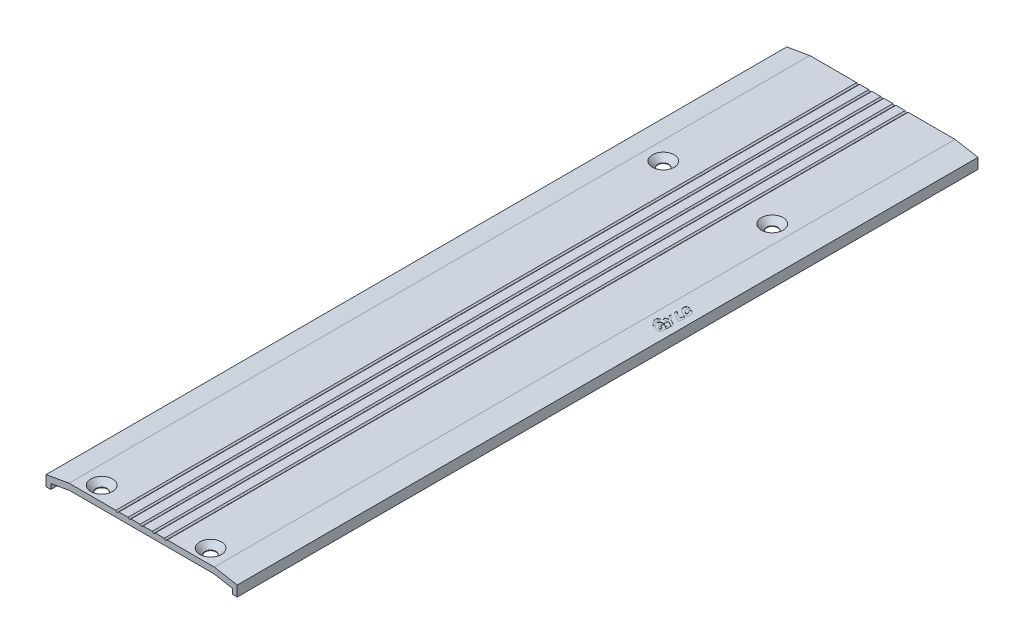
SolidWorks part; units mm, degrees
material "GY-D-79MG 型材"
ref_plane "前视" through (0, 0, 0) normal (0, 0, 1) x (1, 0, 0)
ref_plane "上视" through (0, 0, 0) normal (0, 1, 0) x (1, 0, 0)
ref_plane "右视" through (0, 0, 0) normal (1, 0, 0) x (0, 0, -1)
sketch "Model" plane through (0, 0, 0) normal (0, 0, 1) x (1, 0, 0)
  line L0 (2831.0922, 745.1016) -> (2821.5922, 743.4265)
  line L1 (2821.5922, 743.4265) -> (2821.5922, 739.1016)
  line L2 (2821.5922, 739.1016) -> (2823.5922, 739.1016)
  line L3 (2823.5922, 739.1016) -> (2823.5922, 741.2406)
  line L4 (2823.5922, 741.2406) -> (2831.3109, 742.6016)
  line L5 (2831.3109, 742.6016) -> (2890.8735, 742.6016)
  line L6 (2890.8735, 742.6016) -> (2898.5922, 741.2406)
  line L7 (2898.5922, 741.2406) -> (2898.5922, 739.1016)
  line L8 (2898.5922, 739.1016) -> (2900.5922, 739.1016)
  line L9 (2900.5922, 739.1016) -> (2900.5922, 743.4265)
  line L10 (2900.5922, 743.4265) -> (2891.0922, 745.1016)
  line L11 (2891.0922, 745.1016) -> (2871.7103, 745.1016)
  line L12 (2871.7103, 745.1016) -> (2871.0922, 744.6016)
  line L13 (2871.0922, 744.6016) -> (2870.4742, 745.1016)
  line L14 (2870.4742, 745.1016) -> (2866.7103, 745.1016)
  line L15 (2866.7103, 745.1016) -> (2866.0922, 744.6016)
  line L16 (2866.0922, 744.6016) -> (2865.4742, 745.1016)
  line L17 (2865.4742, 745.1016) -> (2861.7103, 745.1016)
  line L18 (2861.7103, 745.1016) -> (2861.0922, 744.6016)
  line L19 (2861.0922, 744.6016) -> (2860.4742, 745.1016)
  line L20 (2860.4742, 745.1016) -> (2856.7103, 745.1016)
  line L21 (2856.7103, 745.1016) -> (2856.0922, 744.6016)
  line L22 (2856.0922, 744.6016) -> (2855.4742, 745.1016)
  line L23 (2855.4742, 745.1016) -> (2851.7103, 745.1016)
  line L24 (2851.7103, 745.1016) -> (2851.0922, 744.6016)
  line L25 (2851.0922, 744.6016) -> (2850.4742, 745.1016)
  line L26 (2850.4742, 745.1016) -> (2831.0922, 745.1016)
extrude "凸台-拉伸1" add sketch "Model" along normal blind 250
sketch "草图1" plane through (214.597, 1217.0399, 0) normal (0.1736, 0.9848, 0) x (0.9848, -0.1736, 0)
  line B0 (2729.0623, -100) -> (2729.0623, -99)
  line B1 (2729.0623, -99) -> (2729.0623, -98)
  line B2 (2729.0623, -98) -> (2729.0623, -97)
  line B3 (2729.0623, -97) -> (2729.0623, -96)
  line B4 (2729.0623, -96) -> (2729.0623, -95)
  line B5 (2729.0623, -95) -> (2729.0623, -94)
  line B6 (2729.0623, -94) -> (2729.0623, -93)
  line B7 (2729.0623, -100) -> (2730.0623, -100)
  line B8 (2730.0623, -100) -> (2731.0623, -100)
  line B9 (2731.0623, -100) -> (2732.0623, -100)
  line B10 (2729.5623, -100) -> (2729.5623, -98)
  line B11 (2730.0623, -100) -> (2730.0623, -97)
  line B12 (2731.0623, -100) -> (2731.0623, -95)
  line B13 (2730.5623, -100) -> (2730.5623, -96)
  line B14 (2731.5623, -100) -> (2731.5623, -94)
  line B15 (2732.0623, -100) -> (2732.0623, -93)
  line B16 (2723.0623, -83) -> (2721.5854, -81.6515) construction
  line B17 (2723.0623, -83) -> (2723.0623, -94) construction
  line B18 (2723.3995, -82.6308) -> (2723.3995, -81.4458)
  line B19 (2723.3995, -82.6308) -> (2723.0623, -83) construction
  line B20 (2723.0623, -83) -> (2722.0509, -84.1077) construction
  line B21 (2723.0623, -83) -> (2723.8008, -83.6743) construction
  line B22 (2729.0623, -98) -> (2729.5623, -98)
  line B23 (2729.0623, -96) -> (2730.5623, -96)
  line B24 (2723.0623, -94) -> (2721.5854, -92.6515) construction
  line B25 (2722.747, -93.2537) -> (2722.6598, -92.2576)
  line B26 (2723.3995, -93.6308) -> (2723.0623, -94) construction
  line B27 (2723.0623, -94) -> (2722.0509, -95.1077) construction
  line B28 (2723.0623, -94) -> (2723.8008, -94.6743) construction
  line B29 (2722.8134, -82.2727) -> (2722.8134, -81.2727)
  line B30 (2724.6368, -93.6308) -> (2724.8524, -93.6308)
  line B31 (2723.0089, -93.9512) -> (2723.0089, -92.2611)
  line B32 (2723.0089, -92.2611) -> (2724.8524, -93.1308)
  line B33 (2724.8524, -93.1308) -> (2724.8524, -93.6308)
  line B34 (2723.0089, -93.9512) -> (2723.4528, -94.1813)
  line B35 (2723.4528, -94.1813) -> (2723.4528, -93.6813)
  line B36 (2729.0623, -93) -> (2729.0623, -92)
  line B37 (2729.0623, -92) -> (2729.0623, -91)
  line B38 (2729.0623, -91) -> (2729.0623, -90)
  line B39 (2732.0623, -100) -> (2733.0623, -100)
  line B40 (2733.0623, -100) -> (2733.0623, -89)
  line B41 (2724.8524, -91.1308) -> (2724.8524, -90.1308)
  line B42 (2724.8524, -91.1308) -> (2722.973, -90.4467)
  line B43 (2722.973, -89.4467) -> (2721.2722, -87.6308)
  line B44 (2721.2722, -87.6308) -> (2721.2722, -88.6308)
  line B45 (2721.2722, -88.6308) -> (2722.2927, -89.7203)
  line B46 (2722.2927, -89.7203) -> (2721.2722, -90.1308)
  line B47 (2721.2722, -90.1308) -> (2721.2722, -91.1308)
  line B48 (2721.2722, -91.1308) -> (2722.973, -90.4467)
  line B49 (2722.973, -89.4467) -> (2724.8524, -90.1308)
  line B50 (2724.8524, -91.1308) -> (2724.8524, -93.1308) construction
  line B51 (2721.2722, -86.442) -> (2724.8524, -88.1308)
  line B52 (2732.5623, -100) -> (2732.5623, -90)
  line B53 (2729.0623, -90) -> (2732.5623, -90)
  line B54 (2724.8524, -88.1308) -> (2724.8524, -85.6308)
  line B55 (2724.8524, -85.6308) -> (2723.948, -85.2041)
  line B56 (2723.948, -85.2041) -> (2723.948, -86.7041)
  line B57 (2723.948, -86.7041) -> (2721.2722, -85.442)
  line B58 (2721.2722, -85.442) -> (2721.2722, -86.442)
  line B59 (2724.8524, -88.1308) -> (2724.8524, -90.1308) construction
  line B60 (2729.0623, -94) -> (2731.5623, -94)
  line B61 (2721.2722, -88.6308) -> (2721.2722, -90.1308) construction
  line B62 (2720.987, -92.6089) -> (2720.8322, -91.621)
  line B63 (2725.2924, -96.379) -> (2725.1376, -95.3911)
  line B64 (2720.9216, -92.7088) -> (2723.0623, -94) construction
  line B65 (2724.0953, -92.2874) -> (2723.0623, -94) construction
  line B66 (2723.0623, -94) -> (2726.0594, -95.8076) construction
  line B67 (2729.0623, -92) -> (2732.5623, -92)
  line B68 (2729.0623, -95) -> (2731.0623, -95)
  line B69 (2729.0623, -90) -> (2729.0623, -89)
  line B70 (2729.0623, -100) -> (2723.0623, -100) construction
  line B71 (2723.0623, -100) -> (2723.0623, -94) construction
  ellipse B72 centre (2723.0623, -83) end of major axis (2722.3238, -82.3257) minor radius 0.5 (2722.8134, -82.2727) -> (2723.3995, -82.6308) ccw
  ellipse B73 centre (2723.0623, -83) end of major axis (2724.5393, -84.3485) minor radius 1.5 (2722.8134, -81.2727) -> (2723.3995, -81.4458) ccw
  ellipse B74 centre (2723.0623, -94) end of major axis (2722.3238, -93.3257) minor radius 0.5 (2722.747, -93.2537) -> (2723.4528, -93.6813) ccw
  ellipse B75 centre (2723.0623, -94) end of major axis (2721.5854, -92.6515) minor radius 1.5 (2722.6598, -92.2576) -> (2724.6368, -93.6308) ccw
  ellipse B76 centre (2723.0623, -94) end of major axis (2720.0653, -92.1924) minor radius 2 (2720.8322, -91.621) -> (2722.0294, -95.7126) ccw
  ellipse B77 centre (2723.0623, -94) end of major axis (2725.2031, -95.2912) minor radius 2 (2720.987, -92.6089) -> (2722.0294, -95.7126) ccw
  ellipse B78 centre (2723.0623, -94) end of major axis (2720.0653, -92.1924) minor radius 2 (2725.2924, -96.379) -> (2724.0953, -92.2874) ccw
  ellipse B79 centre (2723.0623, -94) end of major axis (2720.9216, -92.7088) minor radius 2 (2725.1376, -95.3911) -> (2724.0953, -92.2874) ccw
sketch_block_instance "块1-1"
sketch_block "块1" parameters "D1"=1, "D2"=70, "D3"=47.602, "D4"=11.302, "D5"=50, "D6"=5, "D7"=15
extrude "切除-拉伸1" cut sketch "草图1" against normal blind 0.1 contours B29 B73 B18 B72 | B57 B58 B51 B54 B55 B56 | B49 B43 B44 B45 B46 B47 B48 B42 B41 | B25 B75 B30 B33 B32 B31 B34 B35 B74 | B77 B62 B76 | B79 B63 B78
sketch "草图4" plane through (0, 0, 250) normal (0, 0, 1) x (1, 0, 0)
  line L27 (2850.4742, 745.1016) -> (2831.0922, 745.1016)
  line L28 (2831.0922, 745.1016) -> (2821.5922, 743.4265)
  line L29 (2821.5922, 743.4265) -> (2821.5922, 739.1016)
  line L30 (2821.5922, 739.1016) -> (2823.5922, 739.1016)
  line L31 (2823.5922, 739.1016) -> (2823.5922, 741.2406)
  line L32 (2823.5922, 741.2406) -> (2831.3109, 742.6016)
  line L33 (2831.3109, 742.6016) -> (2890.8735, 742.6016)
  line L34 (2890.8735, 742.6016) -> (2898.5922, 741.2406)
  line L35 (2898.5922, 741.2406) -> (2898.5922, 739.1016)
  line L36 (2898.5922, 739.1016) -> (2900.5922, 739.1016)
  line L37 (2900.5922, 739.1016) -> (2900.5922, 743.4265)
  line L38 (2900.5922, 743.4265) -> (2891.0922, 745.1016)
  line L39 (2891.0922, 745.1016) -> (2871.7103, 745.1016)
  line L40 (2871.7103, 745.1016) -> (2871.0922, 744.6016)
  line L41 (2871.0922, 744.6016) -> (2870.4742, 745.1016)
  line L42 (2870.4742, 745.1016) -> (2866.7103, 745.1016)
  line L43 (2866.7103, 745.1016) -> (2866.0922, 744.6016)
  line L44 (2866.0922, 744.6016) -> (2865.4742, 745.1016)
  line L45 (2865.4742, 745.1016) -> (2861.7103, 745.1016)
  line L46 (2861.7103, 745.1016) -> (2861.0922, 744.6016)
  line L47 (2861.0922, 744.6016) -> (2860.4742, 745.1016)
  line L48 (2860.4742, 745.1016) -> (2856.7103, 745.1016)
  line L49 (2856.7103, 745.1016) -> (2856.0922, 744.6016)
  line L50 (2856.0922, 744.6016) -> (2855.4742, 745.1016)
  line L51 (2855.4742, 745.1016) -> (2851.7103, 745.1016)
  line L52 (2851.7103, 745.1016) -> (2851.0922, 744.6016)
  line L53 (2851.0922, 744.6016) -> (2850.4742, 745.1016)
  line L54 (2850.4742, 745.1016) -> (2831.0922, 745.1016)
  line L55 (2831.0922, 745.1016) -> (2821.5922, 743.4265)
  line L56 (2821.5922, 743.4265) -> (2821.5922, 739.1016)
  line L57 (2821.5922, 739.1016) -> (2823.5922, 739.1016)
  line L58 (2823.5922, 739.1016) -> (2823.5922, 741.2406)
  line L59 (2823.5922, 741.2406) -> (2831.3109, 742.6016)
  line L60 (2831.3109, 742.6016) -> (2890.8735, 742.6016)
  line L61 (2890.8735, 742.6016) -> (2898.5922, 741.2406)
  line L62 (2898.5922, 741.2406) -> (2898.5922, 739.1016)
  line L63 (2898.5922, 739.1016) -> (2900.5922, 739.1016)
  line L64 (2900.5922, 739.1016) -> (2900.5922, 743.4265)
  line L65 (2900.5922, 743.4265) -> (2891.0922, 745.1016)
  line L66 (2891.0922, 745.1016) -> (2871.7103, 745.1016)
  line L67 (2871.7103, 745.1016) -> (2871.0922, 744.6016)
  line L68 (2871.0922, 744.6016) -> (2870.4742, 745.1016)
  line L69 (2870.4742, 745.1016) -> (2866.7103, 745.1016)
  line L70 (2866.7103, 745.1016) -> (2866.0922, 744.6016)
  line L71 (2866.0922, 744.6016) -> (2865.4742, 745.1016)
  line L72 (2865.4742, 745.1016) -> (2861.7103, 745.1016)
  line L73 (2861.7103, 745.1016) -> (2861.0922, 744.6016)
  line L74 (2861.0922, 744.6016) -> (2860.4742, 745.1016)
  line L75 (2860.4742, 745.1016) -> (2856.7103, 745.1016)
  line L76 (2856.7103, 745.1016) -> (2856.0922, 744.6016)
  line L77 (2856.0922, 744.6016) -> (2855.4742, 745.1016)
  line L78 (2855.4742, 745.1016) -> (2851.7103, 745.1016)
  line L79 (2851.7103, 745.1016) -> (2851.0922, 744.6016)
  line L80 (2851.0922, 744.6016) -> (2850.4742, 745.1016)
  dimension "D1" = 0
extrude "凸台-拉伸2" add sketch "草图4" along normal blind 23
sketch "草图5" plane through (0, 0, 0) normal (0, 0, -1) x (-1, 0, 0)
  line L27 (-2831.0922, 745.1016) -> (-2850.4742, 745.1016)
  line L28 (-2850.4742, 745.1016) -> (-2851.0922, 744.6016)
  line L29 (-2851.0922, 744.6016) -> (-2851.7103, 745.1016)
  line L30 (-2851.7103, 745.1016) -> (-2855.4742, 745.1016)
  line L31 (-2855.4742, 745.1016) -> (-2856.0922, 744.6016)
  line L32 (-2856.0922, 744.6016) -> (-2856.7103, 745.1016)
  line L33 (-2856.7103, 745.1016) -> (-2860.4742, 745.1016)
  line L34 (-2860.4742, 745.1016) -> (-2861.0922, 744.6016)
  line L35 (-2861.0922, 744.6016) -> (-2861.7103, 745.1016)
  line L36 (-2861.7103, 745.1016) -> (-2865.4742, 745.1016)
  line L37 (-2865.4742, 745.1016) -> (-2866.0922, 744.6016)
  line L38 (-2866.0922, 744.6016) -> (-2866.7103, 745.1016)
  line L39 (-2866.7103, 745.1016) -> (-2870.4742, 745.1016)
  line L40 (-2870.4742, 745.1016) -> (-2871.0922, 744.6016)
  line L41 (-2871.0922, 744.6016) -> (-2871.7103, 745.1016)
  line L42 (-2871.7103, 745.1016) -> (-2891.0922, 745.1016)
  line L43 (-2891.0922, 745.1016) -> (-2900.5922, 743.4265)
  line L44 (-2900.5922, 743.4265) -> (-2900.5922, 739.1016)
  line L45 (-2900.5922, 739.1016) -> (-2898.5922, 739.1016)
  line L46 (-2898.5922, 739.1016) -> (-2898.5922, 741.2406)
  line L47 (-2898.5922, 741.2406) -> (-2890.8735, 742.6016)
  line L48 (-2890.8735, 742.6016) -> (-2831.3109, 742.6016)
  line L49 (-2831.3109, 742.6016) -> (-2823.5922, 741.2406)
  line L50 (-2823.5922, 741.2406) -> (-2823.5922, 739.1016)
  line L51 (-2823.5922, 739.1016) -> (-2821.5922, 739.1016)
  line L52 (-2821.5922, 739.1016) -> (-2821.5922, 743.4265)
  line L53 (-2821.5922, 743.4265) -> (-2831.0922, 745.1016)
  line L54 (-2831.0922, 745.1016) -> (-2850.4742, 745.1016)
  line L55 (-2850.4742, 745.1016) -> (-2851.0922, 744.6016)
  line L56 (-2851.0922, 744.6016) -> (-2851.7103, 745.1016)
  line L57 (-2851.7103, 745.1016) -> (-2855.4742, 745.1016)
  line L58 (-2855.4742, 745.1016) -> (-2856.0922, 744.6016)
  line L59 (-2856.0922, 744.6016) -> (-2856.7103, 745.1016)
  line L60 (-2856.7103, 745.1016) -> (-2860.4742, 745.1016)
  line L61 (-2860.4742, 745.1016) -> (-2861.0922, 744.6016)
  line L62 (-2861.0922, 744.6016) -> (-2861.7103, 745.1016)
  line L63 (-2861.7103, 745.1016) -> (-2865.4742, 745.1016)
  line L64 (-2865.4742, 745.1016) -> (-2866.0922, 744.6016)
  line L65 (-2866.0922, 744.6016) -> (-2866.7103, 745.1016)
  line L66 (-2866.7103, 745.1016) -> (-2870.4742, 745.1016)
  line L67 (-2870.4742, 745.1016) -> (-2871.0922, 744.6016)
  line L68 (-2871.0922, 744.6016) -> (-2871.7103, 745.1016)
  line L69 (-2871.7103, 745.1016) -> (-2891.0922, 745.1016)
  line L70 (-2891.0922, 745.1016) -> (-2900.5922, 743.4265)
  line L71 (-2900.5922, 743.4265) -> (-2900.5922, 739.1016)
  line L72 (-2900.5922, 739.1016) -> (-2898.5922, 739.1016)
  line L73 (-2898.5922, 739.1016) -> (-2898.5922, 741.2406)
  line L74 (-2898.5922, 741.2406) -> (-2890.8735, 742.6016)
  line L75 (-2890.8735, 742.6016) -> (-2831.3109, 742.6016)
  line L76 (-2831.3109, 742.6016) -> (-2823.5922, 741.2406)
  line L77 (-2823.5922, 741.2406) -> (-2823.5922, 739.1016)
  line L78 (-2823.5922, 739.1016) -> (-2821.5922, 739.1016)
  line L79 (-2821.5922, 739.1016) -> (-2821.5922, 743.4265)
  line L80 (-2821.5922, 743.4265) -> (-2831.0922, 745.1016)
  dimension "D1" = 0
extrude "凸台-拉伸3" add sketch "草图5" along normal blind 23
hole_wizard "打孔尺寸(%根据)开槽半沉头木螺钉的类型0" positions "草图8" profile "草图9" countersink size "M4" standard "GB" end condition through all
sketch "草图8" plane through (0, 745.1016, 0) normal (0, 1, 0) x (1, 0, 0)
  point P23 (2883.5922, -267)
  point P26 (2838.5922, -267)
  point P30 (2838.5922, -35)
  point P33 (2883.5922, -35)
sketch "草图9" plane through (2883.5922, 745.1016, 267) normal (1, 0, 0) x (0, 0, 1)
  line L0 (0, 0) -> (0, 6)
  line L1 (0, 6) -> (2.25, 6)
  line L2 (2.25, 6) -> (2.25, 2.25)
  line L3 (2.25, 2.25) -> (4.5, 0)
  line L5 (4.5, 0) -> (0, 0)
  line L6 (-2.25, 2.25) -> (-4.5, 0) construction
  line L11 (0, -6.35) -> (0, 107.95) construction
  dimension "通孔孔直径" = 4.5
  dimension "通孔孔深度" = 6
  dimension "近端锥形沉头孔直径" = 9
  dimension "近端锥形沉头孔角度" = 90
sketch "草图10" plane through (0, 0, -23) normal (0, 0, -1) x (-1, 0, 0)
  line L27 (-2821.5922, 743.4265) -> (-2831.0922, 745.1016)
  line L28 (-2831.0922, 745.1016) -> (-2850.4742, 745.1016)
  line L29 (-2850.4742, 745.1016) -> (-2851.0922, 744.6016)
  line L30 (-2851.0922, 744.6016) -> (-2851.7103, 745.1016)
  line L31 (-2851.7103, 745.1016) -> (-2855.4742, 745.1016)
  line L32 (-2855.4742, 745.1016) -> (-2856.0922, 744.6016)
  line L33 (-2856.0922, 744.6016) -> (-2856.7103, 745.1016)
  line L34 (-2856.7103, 745.1016) -> (-2860.4742, 745.1016)
  line L35 (-2860.4742, 745.1016) -> (-2861.0922, 744.6016)
  line L36 (-2861.0922, 744.6016) -> (-2861.7103, 745.1016)
  line L37 (-2861.7103, 745.1016) -> (-2865.4742, 745.1016)
  line L38 (-2865.4742, 745.1016) -> (-2866.0922, 744.6016)
  line L39 (-2866.0922, 744.6016) -> (-2866.7103, 745.1016)
  line L40 (-2866.7103, 745.1016) -> (-2870.4742, 745.1016)
  line L41 (-2870.4742, 745.1016) -> (-2871.0922, 744.6016)
  line L42 (-2871.0922, 744.6016) -> (-2871.7103, 745.1016)
  line L43 (-2871.7103, 745.1016) -> (-2891.0922, 745.1016)
  line L44 (-2891.0922, 745.1016) -> (-2900.5922, 743.4265)
  line L45 (-2900.5922, 743.4265) -> (-2900.5922, 739.1016)
  line L46 (-2900.5922, 739.1016) -> (-2898.5922, 739.1016)
  line L47 (-2898.5922, 739.1016) -> (-2898.5922, 741.2406)
  line L48 (-2898.5922, 741.2406) -> (-2890.8735, 742.6016)
  line L49 (-2890.8735, 742.6016) -> (-2831.3109, 742.6016)
  line L50 (-2831.3109, 742.6016) -> (-2823.5922, 741.2406)
  line L51 (-2823.5922, 741.2406) -> (-2823.5922, 739.1016)
  line L52 (-2823.5922, 739.1016) -> (-2821.5922, 739.1016)
  line L53 (-2821.5922, 739.1016) -> (-2821.5922, 743.4265)
  line L54 (-2821.5922, 743.4265) -> (-2831.0922, 745.1016)
  line L55 (-2831.0922, 745.1016) -> (-2850.4742, 745.1016)
  line L56 (-2850.4742, 745.1016) -> (-2851.0922, 744.6016)
  line L57 (-2851.0922, 744.6016) -> (-2851.7103, 745.1016)
  line L58 (-2851.7103, 745.1016) -> (-2855.4742, 745.1016)
  line L59 (-2855.4742, 745.1016) -> (-2856.0922, 744.6016)
  line L60 (-2856.0922, 744.6016) -> (-2856.7103, 745.1016)
  line L61 (-2856.7103, 745.1016) -> (-2860.4742, 745.1016)
  line L62 (-2860.4742, 745.1016) -> (-2861.0922, 744.6016)
  line L63 (-2861.0922, 744.6016) -> (-2861.7103, 745.1016)
  line L64 (-2861.7103, 745.1016) -> (-2865.4742, 745.1016)
  line L65 (-2865.4742, 745.1016) -> (-2866.0922, 744.6016)
  line L66 (-2866.0922, 744.6016) -> (-2866.7103, 745.1016)
  line L67 (-2866.7103, 745.1016) -> (-2870.4742, 745.1016)
  line L68 (-2870.4742, 745.1016) -> (-2871.0922, 744.6016)
  line L69 (-2871.0922, 744.6016) -> (-2871.7103, 745.1016)
  line L70 (-2871.7103, 745.1016) -> (-2891.0922, 745.1016)
  line L71 (-2891.0922, 745.1016) -> (-2900.5922, 743.4265)
  line L72 (-2900.5922, 743.4265) -> (-2900.5922, 739.1016)
  line L73 (-2900.5922, 739.1016) -> (-2898.5922, 739.1016)
  line L74 (-2898.5922, 739.1016) -> (-2898.5922, 741.2406)
  line L75 (-2898.5922, 741.2406) -> (-2890.8735, 742.6016)
  line L76 (-2890.8735, 742.6016) -> (-2831.3109, 742.6016)
  line L77 (-2831.3109, 742.6016) -> (-2823.5922, 741.2406)
  line L78 (-2823.5922, 741.2406) -> (-2823.5922, 739.1016)
  line L79 (-2823.5922, 739.1016) -> (-2821.5922, 739.1016)
  line L80 (-2821.5922, 739.1016) -> (-2821.5922, 743.4265)
  dimension "D1" = 0
extrude "凸台-拉伸4" add sketch "草图10" along normal blind 10
